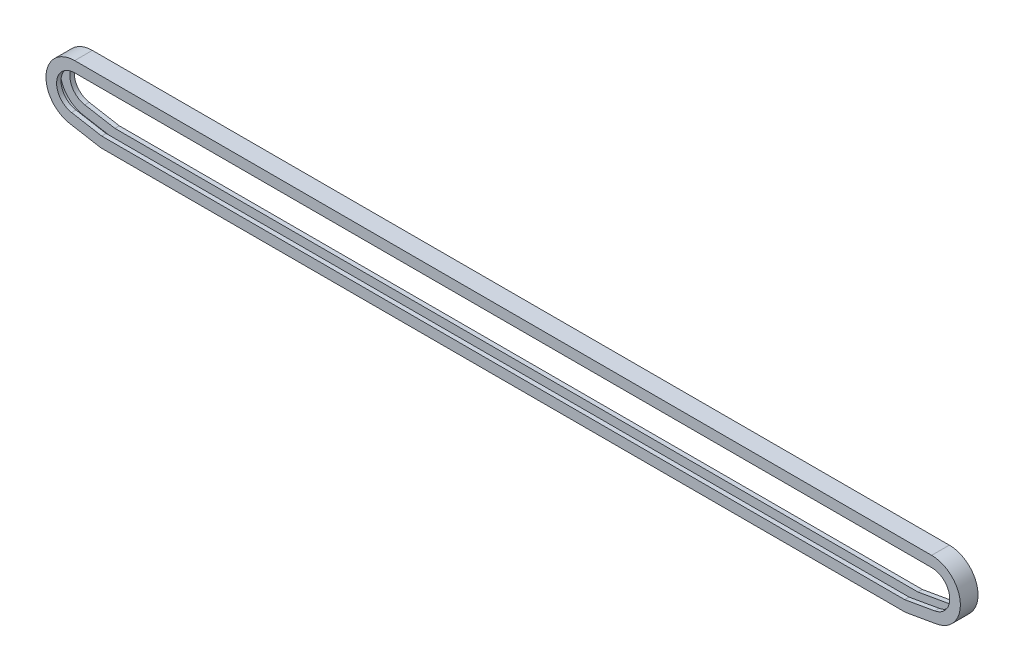
SolidWorks part; units mm, degrees
ref_plane "Front Plane" through (0, 0, 0) normal (0, 0, 1) x (1, 0, 0)
ref_plane "Top Plane" through (0, 0, 0) normal (0, 1, 0) x (1, 0, 0)
ref_plane "Right Plane" through (0, 0, 0) normal (1, 0, 0) x (0, 0, -1)
sketch "Sketch2" plane through (0, 0, 0) normal (0, 0, 1) x (1, 0, 0)
  line L0 (485, 0) -> (-485, 0) construction
  line L1 (0, 0) -> (0, -32.1986) construction
  line L2 (-455, -32.1986) -> (-489.6017, -26.0974) construction
  line L3 (455, -32.1986) -> (489.6017, -26.0974) construction
  line L4 (-485, 26.5) -> (485, 26.5) construction
  line L5 (-455, -32.1986) -> (455, -32.1986) construction
  line L6 (-485, 0) -> (-489.6017, -26.0974) construction
  line L7 (-485, 32.5) -> (485, 32.5)
  line L8 (455.5249, -38.1986) -> (490.6436, -32.0063)
  line L9 (-455.5249, -38.1986) -> (455.5249, -38.1986)
  line L10 (-455.5249, -38.1986) -> (-490.6436, -32.0063)
  line L11 (-485, 20.5) -> (485, 20.5)
  line L12 (454.4751, -26.1986) -> (488.5598, -20.1886)
  line L13 (-454.4751, -26.1986) -> (454.4751, -26.1986)
  line L14 (-454.4751, -26.1986) -> (-488.5598, -20.1886)
  arc A0 (-485, 26.5) -> (-489.6017, -26.0974) centre (-485, 0) ccw construction
  arc A1 (485, 26.5) -> (489.6017, -26.0974) centre (485, 0) cw construction
  arc A2 (485, 32.5) -> (490.6436, -32.0063) centre (485, 0) cw
  arc A3 (-485, 32.5) -> (-490.6436, -32.0063) centre (-485, 0) ccw
  arc A4 (485, 20.5) -> (488.5598, -20.1886) centre (485, 0) cw
  arc A5 (-485, 20.5) -> (-488.5598, -20.1886) centre (-485, 0) ccw
  point P6 (0, 0)
  dimension "D1" = 53
  dimension "D7" = 32.5
  dimension "D8" = 20.5
  dimension "D2" = 970
  dimension "D3" = 30
  dimension "D4" = 100
  dimension "D5" = 6
  dimension "D6" = 6
extrude "Boss-Extrude1" add sketch "Sketch2" along normal mid plane 20
sketch "Sketch8" plane through (0, 0, 0) normal (0, 0, 1) x (1, 0, 0)
  line L18 (455.4374, -37.1986) -> (490.4699, -31.0214)
  line L19 (-455.4374, -37.1986) -> (455.4374, -37.1986)
  line L20 (-490.4699, -31.0214) -> (-455.4374, -37.1986)
  line L21 (485, 31.5) -> (-485, 31.5)
  line L22 (455.4374, -37.1986) -> (490.4699, -31.0214)
  line L23 (-455.4374, -37.1986) -> (455.4374, -37.1986)
  line L24 (-490.4699, -31.0214) -> (-455.4374, -37.1986)
  line L25 (485, 31.5) -> (-485, 31.5)
  arc A12 (490.4699, -31.0214) -> (485, 31.5) centre (485, 0) ccw
  arc A13 (-485, 31.5) -> (-490.4699, -31.0214) centre (-485, 0) ccw
  arc A14 (490.4699, -31.0214) -> (485, 31.5) centre (485, 0) ccw
  arc A15 (-485, 31.5) -> (-490.4699, -31.0214) centre (-485, 0) ccw
  dimension "D1" = 1
extrude "Cut-Extrude1" cut sketch "Sketch8" against normal mid plane 10
